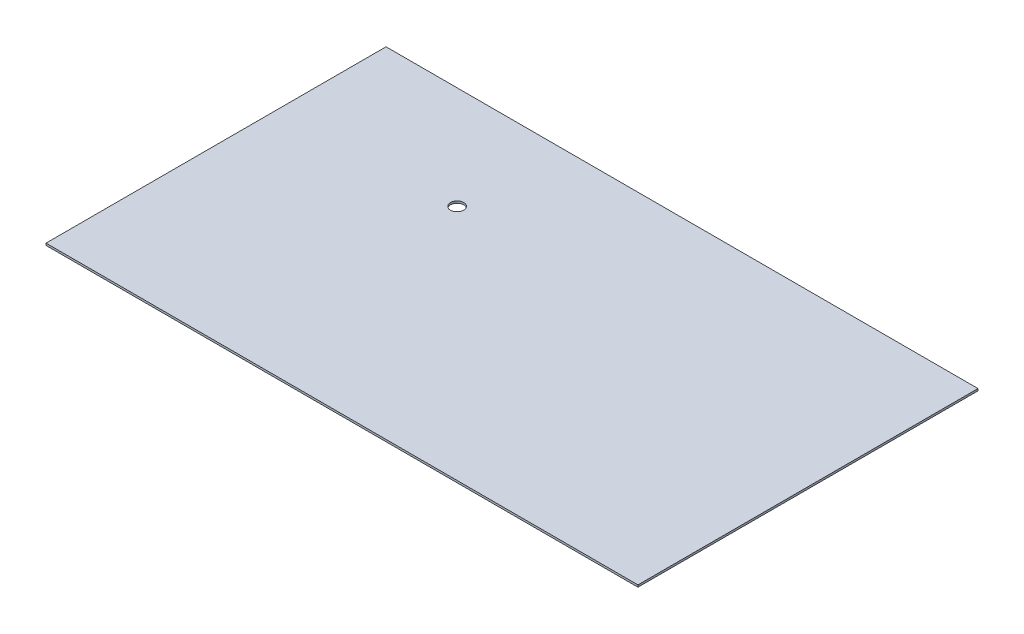
SolidWorks part; units mm, degrees
material "A3"
ref_plane "前视基准面" through (0, 0, 0) normal (0, 0, 1) x (1, 0, 0)
ref_plane "上视基准面" through (0, 0, 0) normal (0, 1, 0) x (1, 0, 0)
ref_plane "右视基准面" through (0, 0, 0) normal (1, 0, 0) x (0, 0, -1)
sketch "草图1" plane through (0, 0, 0) normal (0, 1, 0) x (1, 0, 0)
  line L0 (-235, 667.5) -> (-235, -667.5) construction
  line L1 (-1162, -667.5) -> (1162, -667.5)
  line L2 (-1162, -667.5) -> (-1162, 667.5)
  line L3 (-1162, 667.5) -> (1162, 667.5)
  line L4 (1162, -667.5) -> (1162, 667.5)
  line L5 (-1162, -667.5) -> (1162, 667.5) construction
  line L6 (-1162, 667.5) -> (1162, -667.5) construction
  line L7 (0, 667.5) -> (0, 0) construction
  line L9 (-1162, 507.5) -> (1162, 507.5) construction
  line L10 (-1162, 337.5) -> (1162, 337.5) construction
  line L11 (-1162, 149.5) -> (1162, 149.5) construction
  circle A2 centre (-480, 264.5) radius 26
  point P0 (0, 0)
  dimension "D8" = 235
  dimension "D9" = 52
  dimension "D11" = 480
  dimension "D1" = 1335
  dimension "D2" = 2324
  dimension "D3" = 160
  dimension "D4" = 330
  dimension "D5" = 188
  dimension "D10" = 403
extrude "凸台-拉伸1" add sketch "草图1" along normal mid plane 8
